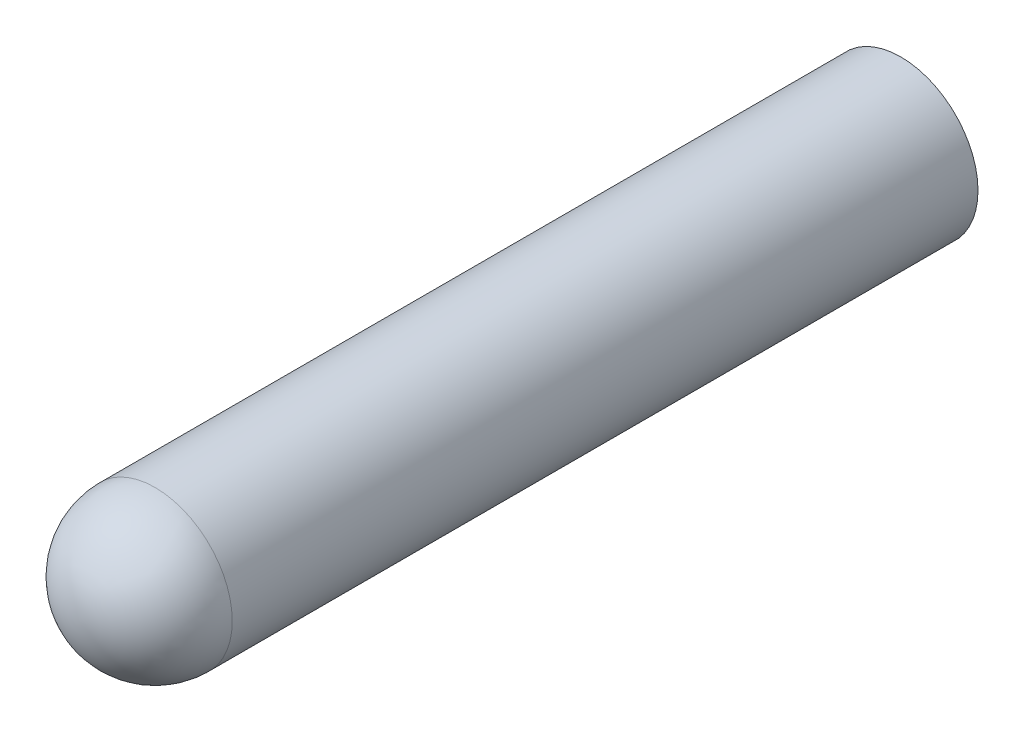
from build123d import *

# Parameters (mm, degrees)
SKETCH1_R           = 1.5
BOSS_EXTRUDE1_DEPTH = 16
FILLET1_R           = 1.5


with BuildPart() as part:
    # Sketch1 → Boss-Extrude1 (new body)
    with BuildSketch(Plane.XY):
        Circle(SKETCH1_R)
    extrude(amount=BOSS_EXTRUDE1_DEPTH)

    # Fillet1
    fillet1_edges = [part.edges().sort_by_distance(p)[0] for p in [
        (-1.5, 0, 16),
    ]]
    fillet(fillet1_edges, radius=FILLET1_R)


solid = part.part
